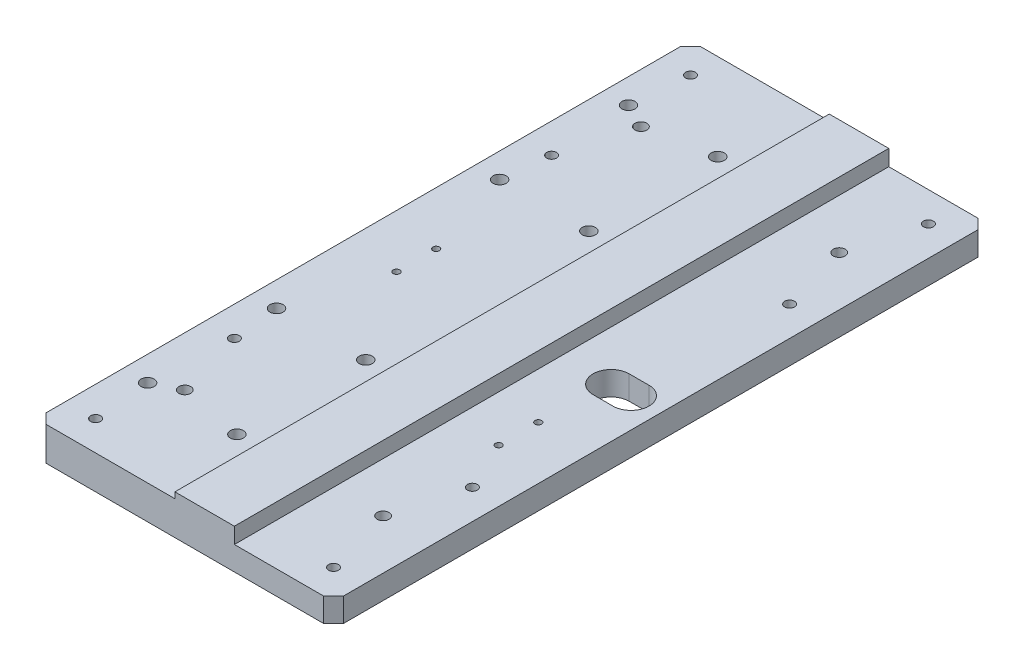
from build123d import *

# Parameters (mm, degrees)
SKETCH_1_W                   = 150
SKETCH_1_H                   = 330
EXTRUDE_1_DEPTH              = 10
SKETCH_2_W                   = 70
SKETCH_2_H                   = 330
CUT_EXTRUDE_1_DEPTH          = 3
SKETCH_3_W                   = 50
SKETCH_3_H                   = 330
CUT_EXTRUDE_2_DEPTH          = 8
MM_1_D                       = 1
HOLE_WIZARD_M6_1_D           = 6.6
HOLE_WIZARD_M6_1_CBORE_D     = 11
HOLE_WIZARD_M6_1_CBORE_DEPTH = 8
MM_0_D                       = 6
HOLE_WIZARD_M6_1_2_D         = 5
CHAMFER_1_SIZE               = 5
CUT_EXTRUDE_3_DEPTH          = 183.345825288
HOLE_WIZARD_M4_1_D           = 3.3


with BuildPart() as part:
    # 草图1 → 凸台-拉伸1 (new, symmetric)
    with BuildSketch(Plane(origin=(0, 0, 0), x_dir=(1, 0, 0), z_dir=(0, 1, 0))):
        Rectangle(SKETCH_1_W, SKETCH_1_H)
    extrude(amount=EXTRUDE_1_DEPTH, both=True)

    # 草图2 → 切除-拉伸1 (cut)
    with BuildSketch(Plane(origin=(0, 10, 0), x_dir=(1, 0, 0), z_dir=(0, 1, 0))):
        with Locations((-40, 0)):
            Rectangle(SKETCH_2_W, SKETCH_2_H)
    extrude(amount=-CUT_EXTRUDE_1_DEPTH, mode=Mode.SUBTRACT)

    # 草图3 → 切除-拉伸2 (cut)
    with BuildSketch(Plane(origin=(0, 10, 0), x_dir=(1, 0, 0), z_dir=(0, 1, 0))):
        with Locations((50, 0)):
            Rectangle(SKETCH_3_W, SKETCH_3_H)
    extrude(amount=-CUT_EXTRUDE_2_DEPTH, mode=Mode.SUBTRACT)

    # 大小mm 暗销孔1 (through all)
    with Locations(Plane(origin=(0, 7, 0), x_dir=(1, 0, 0), z_dir=(0, 1, 0))):
        with Locations((-62.500006208, 121.250006208), (-17.500006208, 121.250006208), (-62.500006208, 56.250006208), (-17.500006208, 56.250006208), (-62.500003219, -56.249995139), (-17.500003219, -56.249995139), (-62.500003219, -121.249995139), (-17.500003219, -121.249995139)):
            Hole(MM_1_D / 2)

    # Hole Wizard M6 _1 (through all)
    with Locations(Plane(origin=(0, -10, 0), x_dir=(-1, 0, 0), z_dir=(0, -1, 0))):
        with Locations((17.500006208, 121.250006208), (62.500006208, 121.250006208), (17.500006208, 56.250006208), (62.500006208, 56.250006208), (17.500003219, -56.249995139), (62.500003219, -56.249995139), (17.500003219, -121.249995139), (62.500003219, -121.249995139)):
            CounterBoreHole(HOLE_WIZARD_M6_1_D / 2, HOLE_WIZARD_M6_1_CBORE_D / 2, HOLE_WIZARD_M6_1_CBORE_DEPTH)

    # 大小mm 暗销孔0 (through all)
    with Locations(Plane(origin=(0, -10, 0), x_dir=(-1, 0, 0), z_dir=(0, -1, 0))):
        with Locations((-50.000000134, 114.999999999), (-50.000000032, -114.999999953), (49.999999866, 114.999999999), (49.999999968, -114.999999953)):
            Hole(MM_0_D / 2)

    # Hole Wizard M6 _1 2 (through all)
    with Locations(Plane(origin=(0, -10, 0), x_dir=(-1, 0, 0), z_dir=(0, -1, 0))):
        with Locations((59.999999968, -149.999999953), (-60.000000032, -149.999999953), (-60.000000032, -79.999999953), (59.999999968, -79.999999953), (59.999999866, 79.999999999), (59.999999866, 149.999999999), (-60.000000134, 149.999999999), (-60.000000134, 79.999999999)):
            Hole(HOLE_WIZARD_M6_1_2_D / 2)

    # 倒角1
    chamfer_1_edges = [part.edges().sort_by_distance(p)[0] for p in [
        (-75, -1.5, -165),
        (-75, -1.5, 165),
        (75, -4, -165),
        (75, -4, 165),
    ]]
    chamfer(chamfer_1_edges, length=CHAMFER_1_SIZE)

    # 草图14 → 切除-拉伸3 (cut, through all)
    with BuildSketch(Plane.XZ.offset(10)):
        with BuildLine():
            Line((50, 9.1), (60, 9.1))
            ThreePointArc((60, 9.1), (69.1, 0), (60, -9.1))
            Line((60, -9.1), (50, -9.1))
            ThreePointArc((50, -9.1), (40.9, 0), (50, 9.1))
        make_face()
    extrude(amount=-CUT_EXTRUDE_3_DEPTH, mode=Mode.SUBTRACT)

    # M4 螺纹孔1 (through all)
    with Locations(Plane(origin=(0, -10, 0), x_dir=(-1, 0, 0), z_dir=(0, -1, 0))):
        with Locations((-48.25000003, -35.000000224), (-48.25000003, -55.000000224), (48.249999938, -10.000000156), (48.249999938, 9.999999844)):
            Hole(HOLE_WIZARD_M4_1_D / 2)


solid = part.part
